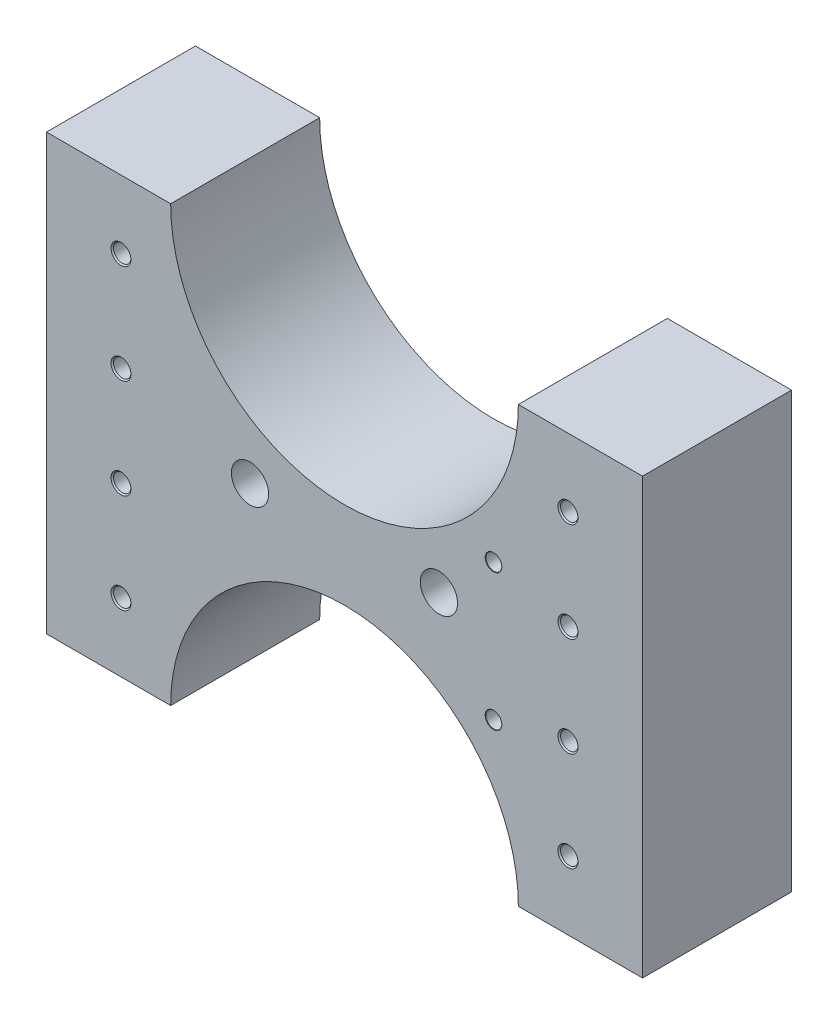
from build123d import *

# Parameters (mm, degrees)
EXTRUDE_1_DEPTH               = 120
HOLE_WIZARD_M16_1_D           = 14
HOLE_WIZARD_M16_1_DEPTH       = 31.793975667
HOLE_WIZARD_M16_1_CSINK_D     = 16.05
HOLE_WIZARD_M16_1_CSINK_ANGLE = 90
HOLE_WIZARD_M16_1_TIP         = 4.206024333
CUT_EXTRUDE_1_DEPTH           = 321.351369593
CUT_EXTRUDE_1_DEPTH_BACK      = 321.351369593
SKETCH_5_R                    = 15
CUT_EXTRUDE_2_DEPTH           = 321.351369593
CUT_EXTRUDE_2_DEPTH_BACK      = 321.351369593
SKETCH_6_R                    = 4
F_1_4_RC_1_AT_2_COUNT         = 2
F_1_4_RC_1_AT_2_PITCH         = 110
F_1_4_RC_2_AT_2_COUNT         = 2
F_1_4_RC_2_AT_2_PITCH         = 110
CUT_EXTRUDE_3_REACH           = 345.165
CUT_EXTRUDE_3_END_RADIUS      = 4
SKETCH_12_R                   = 4
SKETCH_14_R                   = 12.5
CUT_EXTRUDE_4_DEPTH           = 44.01


with BuildPart() as part:
    # 草图1 → 凸台-拉伸1 (new body)
    with BuildSketch(Plane.XY):
        with BuildLine():
            Line((-140, -175), (-240, -175))
            Line((-240, -175), (-240, 175))
            Line((-240, 175), (-140, 175))
            ThreePointArc((-140, 175), (0, 35), (140, 175))
            Line((140, 175), (240, 175))
            Line((240, 175), (240, -175))
            Line((240, -175), (140, -175))
            ThreePointArc((140, -175), (0, -35), (-140, -175))
        make_face()
    extrude(amount=EXTRUDE_1_DEPTH)

    # M16 螺纹孔1
    with Locations(Plane.XY.offset(120)):
        with Locations((-180, 120), (-180, 40), (-180, -40), (-180, -120), (180, -120), (180, -40), (180, 40), (180, 120)):
            CounterSinkHole(HOLE_WIZARD_M16_1_D / 2, HOLE_WIZARD_M16_1_CSINK_D / 2, depth=HOLE_WIZARD_M16_1_DEPTH, counter_sink_angle=HOLE_WIZARD_M16_1_CSINK_ANGLE)
            with Locations((0, 0, -(HOLE_WIZARD_M16_1_DEPTH + HOLE_WIZARD_M16_1_TIP / 2))):  # 118° drill point
                Cone(0, HOLE_WIZARD_M16_1_D / 2, HOLE_WIZARD_M16_1_TIP, mode=Mode.SUBTRACT)

    # 草图5 → 切除-拉伸1 (cut, two sides: drawn at the far end of the back side and taken through both)
    with BuildSketch(Plane.XY.offset(120).offset(-CUT_EXTRUDE_1_DEPTH_BACK)):
        with Locations((-76.071287113, 11.864598333)):
            Circle(SKETCH_5_R)
        with Locations((76.071287113, 11.864598333)):
            Circle(SKETCH_5_R)
    extrude(amount=CUT_EXTRUDE_1_DEPTH + CUT_EXTRUDE_1_DEPTH_BACK, mode=Mode.SUBTRACT)

    # 草图6 → 切除-拉伸2 (cut, two sides: drawn at the far end of the back side and taken through both)
    with BuildSketch(Plane.XY.offset(120).offset(-CUT_EXTRUDE_2_DEPTH_BACK)):
        with Locations((120, 55)):
            Circle(SKETCH_6_R)
        with Locations((120, -55)):
            Circle(SKETCH_6_R)
    extrude(amount=CUT_EXTRUDE_2_DEPTH + CUT_EXTRUDE_2_DEPTH_BACK, mode=Mode.SUBTRACT)

    # 草图8 → 1/4 Rc 螺纹孔1 (revolve, cut)
    with BuildSketch(Plane(origin=(120, 55, 120), x_dir=(0, -1, 0), z_dir=(1, 0, 0))):
        Polygon((0, 0), (0, 20), (5.35, 16.785395688), (5.35, 20), (5.818578894, 20), (6.4349495, 0.2550505), (6.69, 0), align=None)
    f_1_4_rc_1 = revolve(axis=Axis((120, 55, 126.35), (0, 0, -1)), mode=Mode.SUBTRACT)

    # 1/4 Rc 螺纹孔1 at 2: 1/4 Rc 螺纹孔1 ×2
    with Locations(*[(0, -i * F_1_4_RC_1_AT_2_PITCH, 0) for i in range(1, F_1_4_RC_1_AT_2_COUNT)]):
        add(f_1_4_rc_1, mode=Mode.SUBTRACT)

    # 草图10 → 1/4 Rc 螺纹孔2 (revolve, cut)
    with BuildSketch(Plane(origin=(120, 55, 0), x_dir=(0, 1, 0), z_dir=(1, 0, 0))):
        Polygon((0, 0), (0, 20), (5.35, 16.785395688), (5.35, 20), (5.818578894, 20), (6.4349495, 0.2550505), (6.69, 0), align=None)
    f_1_4_rc_2 = revolve(axis=Axis((120, 55, -6.35), (0, 0, 1)), mode=Mode.SUBTRACT)

    # 1/4 Rc 螺纹孔2 at 2: 1/4 Rc 螺纹孔2 ×2
    with Locations(*[(0, -i * F_1_4_RC_2_AT_2_PITCH, 0) for i in range(1, F_1_4_RC_2_AT_2_COUNT)]):
        add(f_1_4_rc_2, mode=Mode.SUBTRACT)

    # 切除-拉伸3: up to this cylinder (the profile starts outside it)
    cut_extrude_3_end = Plane(origin=(120, -55, 60), z_dir=(0, 0, 1)) * Cylinder(CUT_EXTRUDE_3_END_RADIUS, 699.33, mode=Mode.PRIVATE)
    # 草图12 → 切除-拉伸3 (cut, up to the surface)
    with BuildSketch(Plane(origin=(-17.5, -17.5, 0), x_dir=(0, 0, -1), z_dir=(-0.7071067811865488, -0.7071067811865464, 0)), mode=Mode.PRIVATE) as cut_extrude_3_sk1:
        with Locations(Location((-60, 123.743686708, 0), (0, 0, 90))):
            Circle(SKETCH_12_R)
    cut_extrude_3_tool1 = extrude(cut_extrude_3_sk1.sketch, amount=-CUT_EXTRUDE_3_REACH, mode=Mode.PRIVATE) - cut_extrude_3_end
    cut_extrude_3 = cut_extrude_3_tool1.solids().sort_by_distance((70, -105, 60))[0]
    add(cut_extrude_3, mode=Mode.SUBTRACT)

    # 草图14 → 切除-拉伸4 (cut)
    with BuildSketch(Plane(origin=(-17.5, -17.5, 0), x_dir=(0, 0, -1), z_dir=(-0.7071067811865488, -0.7071067811865464, 0))):
        with Locations(Location((-60, 123.743686708, 0), (0, 0, 90))):
            Circle(SKETCH_14_R)
    cut_extrude_4 = extrude(amount=-CUT_EXTRUDE_4_DEPTH, mode=Mode.SUBTRACT)

    # 镜向1: 切除-拉伸3, 切除-拉伸4 across plane
    add(cut_extrude_3.mirror(Plane.ZX), mode=Mode.SUBTRACT)
    add(cut_extrude_4.mirror(Plane.ZX), mode=Mode.SUBTRACT)


solid = part.part
